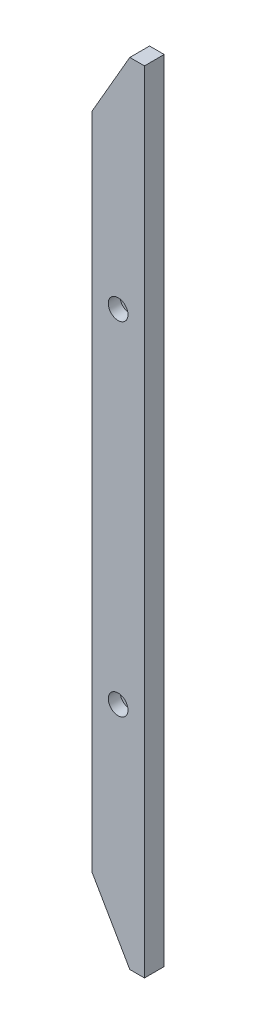
from build123d import *

# Parameters (mm, degrees)
SKETCH_1_W                = 40
SKETCH_1_H                = 600
EXTRUDE_1_DEPTH           = 15
HOLE_WIZARD_1_D           = 9
HOLE_WIZARD_1_CBORE_D     = 15
HOLE_WIZARD_1_CBORE_DEPTH = 9
CHAMFER_1_SIZE            = 50
CHAMFER_1_SIZE2           = 28.867513459


with BuildPart() as part:
    # 草图1 → 凸台-拉伸1 (new body)
    with BuildSketch(Plane.XY):
        Rectangle(SKETCH_1_W, SKETCH_1_H)
    extrude(amount=EXTRUDE_1_DEPTH)

    # 打孔尺寸(%根据)内六角圆柱头螺钉的类型1 (through all)
    with Locations(Plane.XY.offset(15)):
        with Locations((0, -130), (0, 130)):
            CounterBoreHole(HOLE_WIZARD_1_D / 2, HOLE_WIZARD_1_CBORE_D / 2, HOLE_WIZARD_1_CBORE_DEPTH)

    # 倒角1
    chamfer_1_edges = [part.edges().sort_by_distance(p)[0] for p in [
        (-20, 300, 7.5),
        (-20, -300, 7.5),
    ]]
    chamfer_1_side = [part.faces().sort_by_distance(p)[0] for p in [
        (-20, 0, 7.5),
    ]]
    chamfer(chamfer_1_edges, length=CHAMFER_1_SIZE, length2=CHAMFER_1_SIZE2, reference=chamfer_1_side[0])


solid = part.part
